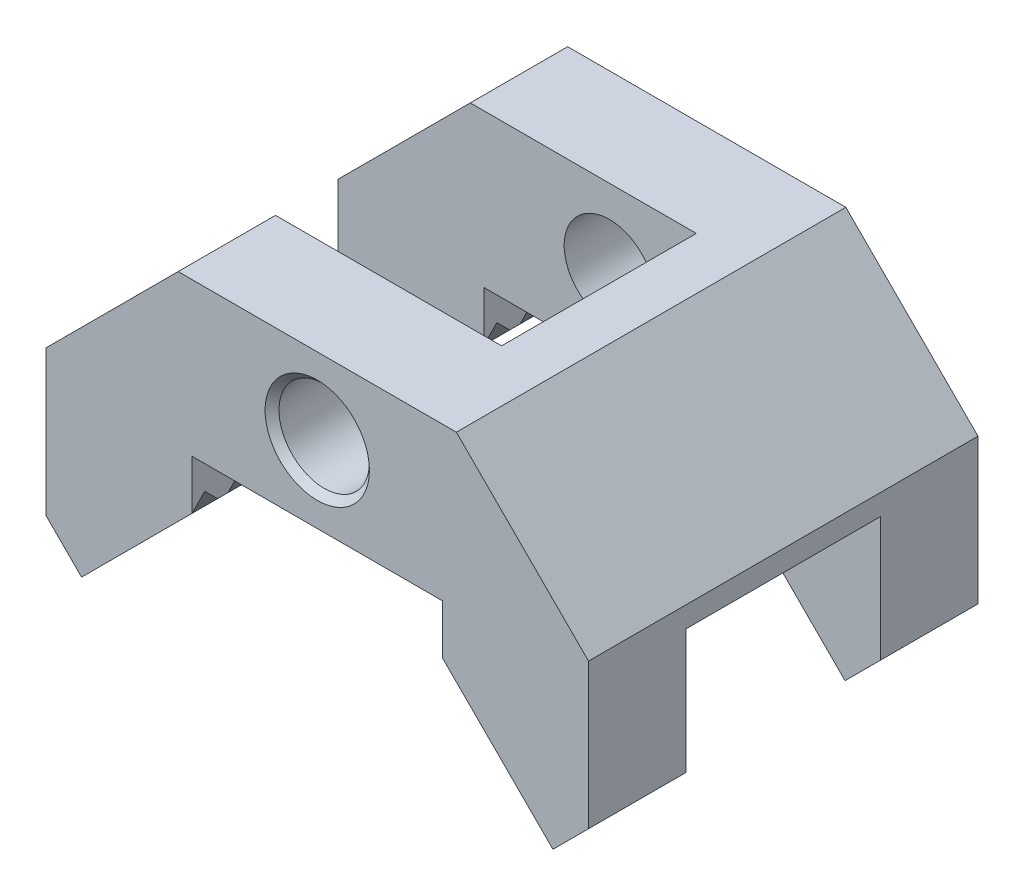
SolidWorks part; units mm, degrees
ref_plane "Front Plane" through (0, 0, 0) normal (0, 0, 1) x (1, 0, 0)
ref_plane "Top Plane" through (0, 0, 0) normal (0, 1, 0) x (1, 0, 0)
ref_plane "Right Plane" through (0, 0, 0) normal (1, 0, 0) x (0, 0, -1)
other "Configuration Table"
sketch "Sketch1" plane through (0, 0, 0) normal (0, 0, 1) x (1, 0, 0)
  line L0 (0, 0) -> (0, 10.4003) construction
  line L1 (20, 11) -> (-20, 11)
  line L2 (-20, 11) -> (-39, -8)
  line L3 (-39, -8) -> (-39, -28.8823)
  line L4 (-39, -28.8823) -> (-33.8848, -33.9975)
  line L5 (-33.8848, -33.9975) -> (-18, -18.1127)
  line L6 (-18, -18.1127) -> (-18, -11)
  line L7 (-18, -11) -> (18, -11)
  line L8 (18, -18.1127) -> (18, -11)
  line L9 (33.8848, -33.9975) -> (18, -18.1127)
  line L10 (39, -28.8823) -> (33.8848, -33.9975)
  line L11 (39, -8) -> (39, -28.8823)
  line L12 (20, 11) -> (39, -8)
  circle A0 centre (0, 0) radius 6.5
  point P13 (0, -11)
  point P18 (0, 11)
  dimension "D1" = 13
  dimension "D2" = 36
  dimension "D3" = 40
  dimension "D4" = 22
  dimension "D5" = 45
  dimension "D6" = 90
  dimension "D7" = 48
  dimension "D8" = 22
  dimension "D9" = 78
  dimension "D10" = 11
extrude "Boss-Extrude1" add sketch "Sketch1" along normal mid plane 56
sketch "Sketch2" plane through (0, 0, 28) normal (0, 0, 1) x (1, 0, 0)
  line L1 (-52.9032, 36.8249) -> (12.5, 36.8249)
  line L2 (-52.9032, 36.8249) -> (-52.9032, -36.8249)
  line L3 (-52.9032, -36.8249) -> (12.5, -36.8249)
  line L4 (12.5, 36.8249) -> (12.5, -36.8249)
  line L5 (-52.9032, 36.8249) -> (12.5, -36.8249) construction
  line L6 (-52.9032, -36.8249) -> (12.5, 36.8249) construction
  point P0 (-20.2016, 0)
  dimension "D1" = 12.5
  dimension "D2" = 65.4032
  dimension "D3" = 73.6498
extrude "Cut-Extrude1" cut sketch "Sketch2" against normal blind 28 from offset 14 offset against normal yes
sketch "Sketch3" plane through (-18, 0, 0) normal (1, 0, 0) x (0, 0, -1)
  line L0 (0, 0) -> (0, -17.4656) construction
  line L1 (14, -18.1127) -> (28, -18.1127) construction
  line L2 (14, -18.1127) -> (17.6667, -18.1127)
  line L3 (14, -18.1127) -> (15.8333, -16.2794)
  line L4 (15.8333, -16.2794) -> (17.6667, -18.1127)
  line L5 (19.1667, -18.1127) -> (22.8333, -18.1127)
  line L6 (19.1667, -18.1127) -> (21, -16.2794)
  line L7 (21, -19.4475) -> (21, -11.9415) construction
  line L8 (22.8333, -18.1127) -> (21, -16.2794)
  line L9 (28, -18.1127) -> (26.1667, -16.2794)
  line L10 (26.1667, -16.2794) -> (24.3333, -18.1127)
  line L11 (24.3333, -18.1127) -> (28, -18.1127)
  dimension "D1" = 1.5
sketch "Sketch5" plane through (-33.9411, -33.9411, 0) normal (-0.7071, -0.7071, 0) x (0, 0, 1)
  line L3 (-22.8333, -0.0797) -> (-19.1667, -0.0797)
  line L4 (-21, 1.2167) -> (-22.8333, -0.0797)
  line L5 (-19.1667, -0.0797) -> (-21, 1.2167)
  line L6 (-22.8333, -0.0797) -> (-19.1667, -0.0797)
  line L7 (-21, 1.2167) -> (-22.8333, -0.0797)
  line L8 (-19.1667, -0.0797) -> (-21, 1.2167)
  line L9 (-17.6667, -0.0797) -> (-14, -0.0797)
  line L10 (-15.8333, 1.2167) -> (-17.6667, -0.0797)
  line L11 (-14, -0.0797) -> (-15.8333, 1.2167)
  line L12 (-17.6667, -0.0797) -> (-14, -0.0797)
  line L13 (-15.8333, 1.2167) -> (-17.6667, -0.0797)
  line L14 (-14, -0.0797) -> (-15.8333, 1.2167)
  line L15 (-24.3333, -0.0797) -> (-26.1667, 1.2167)
  line L16 (-28, -0.0797) -> (-24.3333, -0.0797)
  line L17 (-26.1667, 1.2167) -> (-28, -0.0797)
  line L18 (-24.3333, -0.0797) -> (-26.1667, 1.2167)
  line L19 (-28, -0.0797) -> (-24.3333, -0.0797)
  line L20 (-26.1667, 1.2167) -> (-28, -0.0797)
  dimension "D1" = 0
  dimension "D2" = 0
  dimension "D3" = 0
extrude "Cut-Extrude2" cut sketch "Sketch5" against normal blind 28
mirror "Mirror1" about plane through (0, 0, 0) normal (0, 0, 1) of "Cut-Extrude2"
mirror "Mirror2" about plane through (0, 0, 0) normal (1, 0, 0) of "Mirror1", "Cut-Extrude2"
chamfer "Chamfer1" distance 1 angle 45 2 edges at (6.5, 0, -28) (6.5, 0, 28)
sketch "Sketch6" plane through (0, 0, 28) normal (0, 0, 1) x (1, 0, 0)
  line L1 (18, -11) -> (46.1471, -11)
  line L2 (18, -11) -> (18, -37.3965)
  line L3 (18, -37.3965) -> (46.1471, -37.3965)
  line L4 (46.1471, -11) -> (46.1471, -37.3965)
  dimension "D1" = 28.1471
  dimension "D2" = 26.3965
extrude "Cut-Extrude3" cut sketch "Sketch6" against normal blind 28 from offset 14
